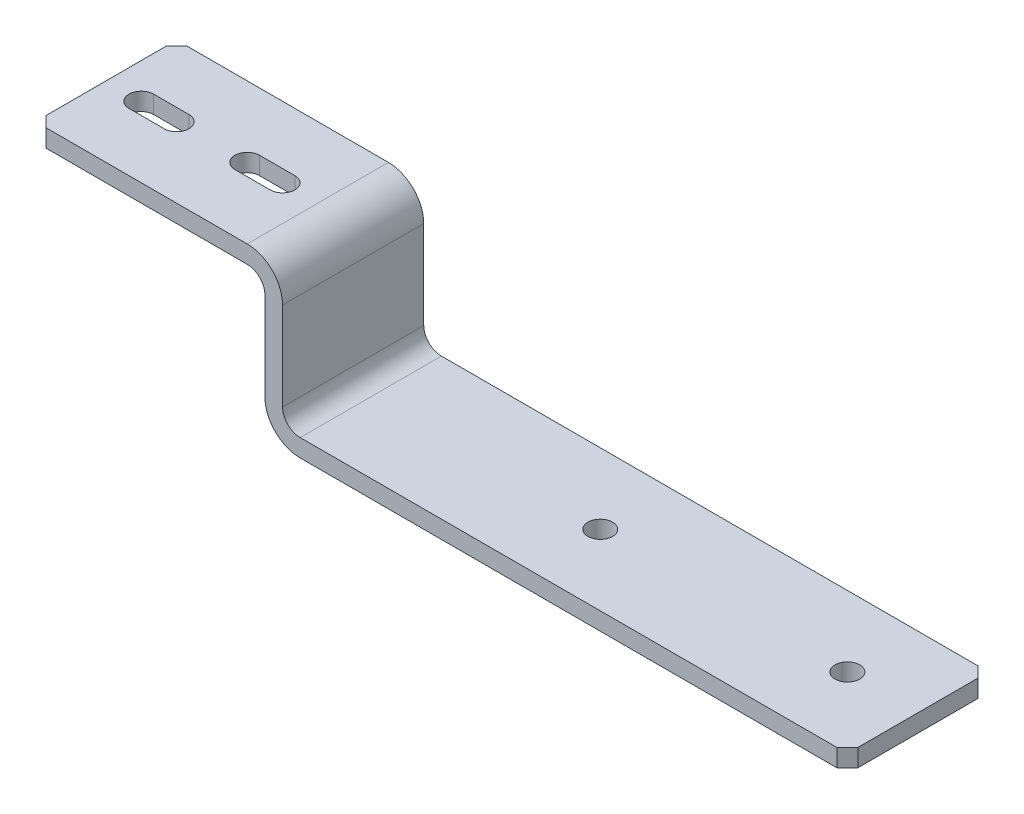
from build123d import *

# Parameters (mm, degrees)
BOSS_EXTRUDE1_DEPTH = 40
CUT_EXTRUDE1_DEPTH  = 40
SKETCH3_R           = 3.5
CUT_EXTRUDE2_DEPTH  = 40
CHAMFER1_SIZE       = 3


with BuildPart() as part:
    # Sketch1 → Boss-Extrude1 (new body)
    with BuildSketch(Plane.XY):
        with BuildLine():
            Line((0, 0), (60, 0))
            ThreePointArc((60, 0), (63.535533906, -1.464466094), (65, -5))
            Line((65, -5), (65, -30))
            ThreePointArc((65, -30), (67.928932188, -37.071067812), (75, -40))
            Line((75, -40), (230, -40))
            Line((230, -40), (230, -35))
            Line((230, -35), (75, -35))
            ThreePointArc((75, -35), (71.464466094, -33.535533906), (70, -30))
            Line((70, -30), (70, -5))
            ThreePointArc((70, -5), (67.071067812, 2.071067812), (60, 5))
            Line((60, 5), (0, 5))
            Line((0, 5), (0, 0))
        make_face()
    extrude(amount=BOSS_EXTRUDE1_DEPTH)

    # Sketch2 → Cut-Extrude1 (cut)
    with BuildSketch(Plane(origin=(0, 5, 0), x_dir=(1, 0, 0), z_dir=(0, 1, 0))):
        with BuildLine():
            Line((10, -16.5), (20, -16.5))
            ThreePointArc((20, -16.5), (23.5, -20), (20, -23.5))
            Line((20, -23.5), (10, -23.5))
            ThreePointArc((10, -23.5), (6.5, -20), (10, -16.5))
        make_face()
        with BuildLine():
            Line((40, -16.5), (50, -16.5))
            ThreePointArc((50, -16.5), (53.5, -20), (50, -23.5))
            Line((50, -23.5), (40, -23.5))
            ThreePointArc((40, -23.5), (36.5, -20), (40, -16.5))
        make_face()
    extrude(amount=-CUT_EXTRUDE1_DEPTH, mode=Mode.SUBTRACT)

    # Sketch3 → Cut-Extrude2 (cut)
    with BuildSketch(Plane(origin=(0, -35, 0), x_dir=(1, 0, 0), z_dir=(0, 1, 0))):
        with Locations(Location((140, -20, 0), (0, 0, 270))):
            Circle(SKETCH3_R)
        with Locations(Location((210, -20, 0), (0, 0, 270))):
            Circle(SKETCH3_R)
    extrude(amount=-CUT_EXTRUDE2_DEPTH, mode=Mode.SUBTRACT)

    # Chamfer1
    chamfer1_edges = [part.edges().sort_by_distance(p)[0] for p in [
        (0, 2.5, 0),
        (230, -37.5, 0),
        (0, 2.5, 40),
        (230, -37.5, 40),
    ]]
    chamfer(chamfer1_edges, length=CHAMFER1_SIZE)


solid = part.part
